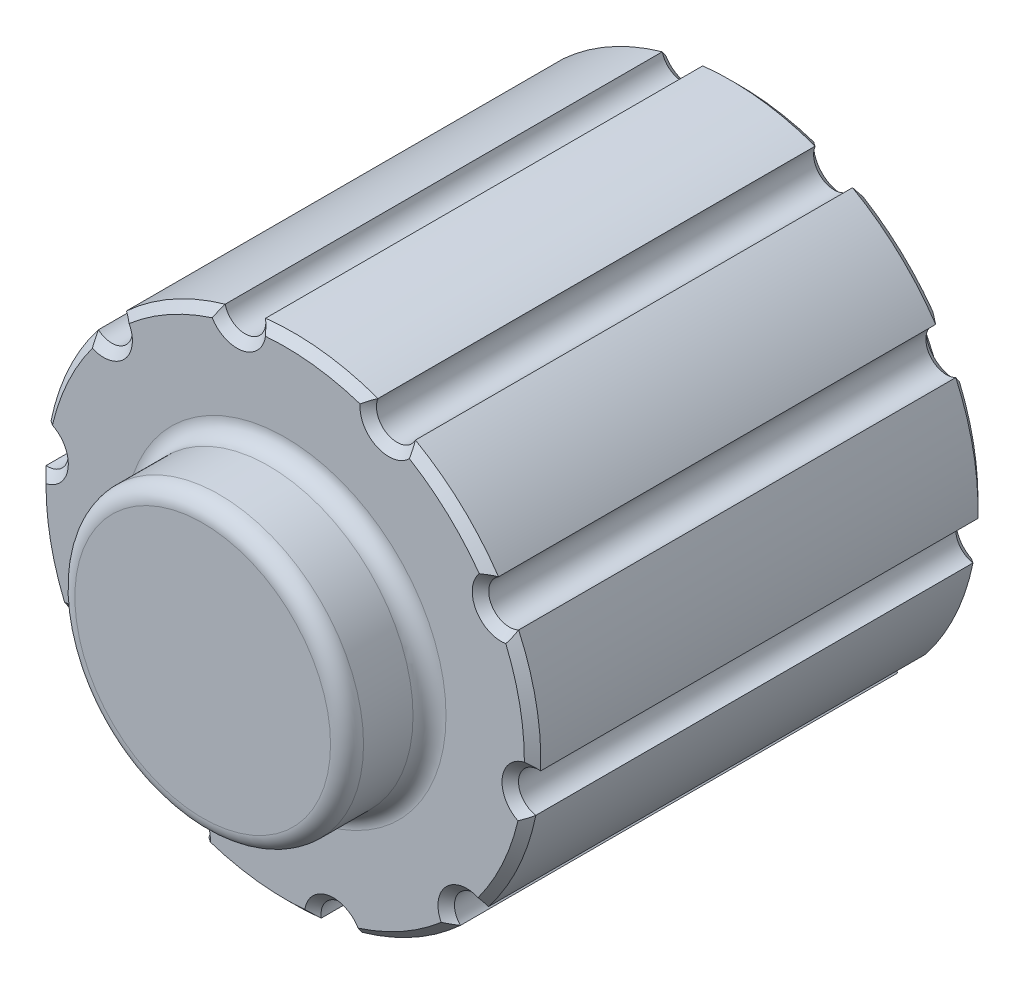
from build123d import *

# Parameters (mm, degrees)
SKETCH1_R           = 20
BOSS_EXTRUDE1_DEPTH = 5
SKETCH2_R           = 30
BOSS_EXTRUDE2_DEPTH = 55
SKETCH3_R           = 2.5
CUT_EXTRUDE1_DEPTH  = 55
CHAMFER1_SIZE       = 1
SKETCH4_R           = 17.5
BOSS_EXTRUDE3_DEPTH = 10
FILLET1_R           = 2


with BuildPart() as part:
    # Sketch1 → Boss-Extrude1 (new body)
    with BuildSketch(Plane.XY):
        with Locations((-119, -40)):
            Circle(SKETCH1_R)
    extrude(amount=BOSS_EXTRUDE1_DEPTH)

    # Sketch2 → Boss-Extrude2 (add)
    with BuildSketch(Plane.XY.offset(5)):
        with Locations((-119, -40)):
            Circle(SKETCH2_R)
    extrude(amount=BOSS_EXTRUDE2_DEPTH)

    # Sketch3 → Cut-Extrude1 (cut)
    with BuildSketch(Plane.XY.offset(60)):
        with Locations((-92.821488811, -25.347848215)):
            Circle(SKETCH3_R)
        with Locations((-89.208820827, -43.533503006)):
            Circle(SKETCH3_R)
        with Locations((-96.975370722, -60.369479748)):
            Circle(SKETCH3_R)
        with Locations((-113.154580412, -69.425007559)):
            Circle(SKETCH3_R)
        with Locations((-131.566541706, -67.241182602)):
            Circle(SKETCH3_R)
        with Locations((-145.178511189, -54.652151785)):
            Circle(SKETCH3_R)
        with Locations((-148.791179173, -36.466496994)):
            Circle(SKETCH3_R)
        with Locations((-141.024629278, -19.630520252)):
            Circle(SKETCH3_R)
        with Locations((-124.845419588, -10.574992441)):
            Circle(SKETCH3_R)
        with Locations((-106.433458294, -12.758817398)):
            Circle(SKETCH3_R)
    extrude(amount=-CUT_EXTRUDE1_DEPTH, mode=Mode.SUBTRACT)

    # Chamfer1
    chamfer1_edges = [part.edges().sort_by_distance(p)[0] for p in [
        (-115.466496994, -10.208820827, 5),
        (-133.652151785, -13.821488811, 5),
        (-146.241182602, -27.433458294, 5),
        (-148.425007559, -45.845419588, 5),
        (-139.369479748, -62.024629278, 5),
        (-122.533503006, -69.791179173, 5),
        (-104.347848215, -66.178511189, 5),
        (-91.758817398, -52.566541706, 5),
        (-89.574992441, -34.154580412, 5),
        (-130.519329897, -64.971084052, 5),
        (-142.99696859, -53.431139136, 5),
        (-146.308580908, -36.760955578, 5),
        (-139.189243504, -21.327976898, 5),
        (-124.358301289, -13.027076404, 5),
        (-98.630520252, -17.975370722, 60),
        (-115.466496994, -10.208820827, 60),
        (-133.652151785, -13.821488811, 60),
        (-146.241182602, -27.433458294, 60),
        (-148.425007559, -45.845419588, 60),
        (-139.369479748, -62.024629278, 60),
        (-122.533503006, -69.791179173, 60),
        (-104.347848215, -66.178511189, 60),
        (-91.758817398, -52.566541706, 60),
        (-89.574992441, -34.154580412, 60),
        (-124.358301289, -13.027076404, 60),
        (-139.189243504, -21.327976898, 60),
        (-146.308580908, -36.760955578, 60),
        (-139, -40, 5),
        (-142.99696859, -53.431139136, 60),
        (-130.519329897, -64.971084052, 60),
        (-113.641698711, -66.972923596, 60),
        (-113.641698711, -66.972923596, 5),
        (-98.810756496, -58.672023102, 60),
        (-98.810756496, -58.672023102, 5),
        (-91.691419092, -43.239044422, 60),
        (-91.691419092, -43.239044422, 5),
        (-107.480670103, -15.028915948, 60),
        (-107.480670103, -15.028915948, 5),
        (-95.00303141, -26.568860864, 60),
        (-95.00303141, -26.568860864, 5),
        (-98.630520252, -17.975370722, 5),
    ]]
    chamfer(chamfer1_edges, length=CHAMFER1_SIZE)

    # Sketch4 → Boss-Extrude3 (add)
    with BuildSketch(Plane.XY.offset(60)):
        with Locations((-119, -40)):
            Circle(SKETCH4_R)
    extrude(amount=BOSS_EXTRUDE3_DEPTH)

    # Fillet1
    fillet1_edges = [part.edges().sort_by_distance(p)[0] for p in [
        (-136.5, -40, 60),
        (-136.5, -40, 70),
    ]]
    fillet(fillet1_edges, radius=FILLET1_R)


solid = part.part
